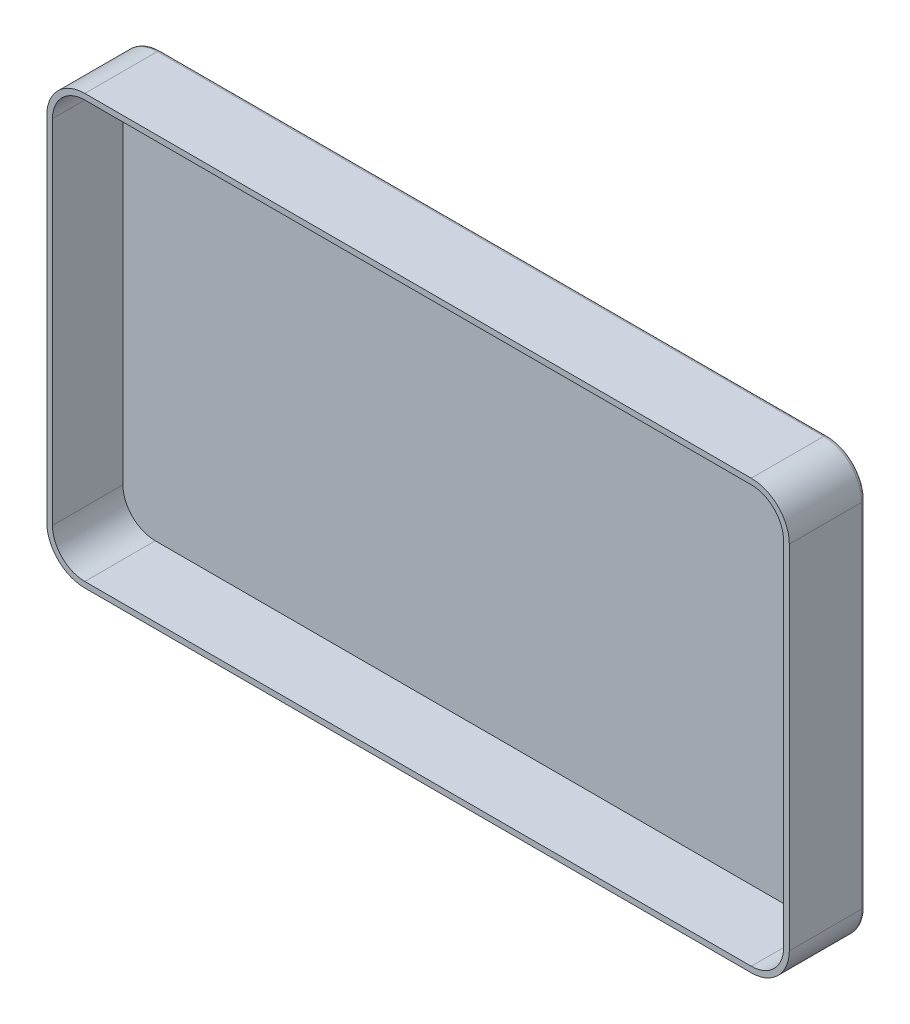
from build123d import *

# Parameters (mm, degrees)
SKETCH_1_W                     = 390
SKETCH_1_H                     = 225
EXTRUDE_1_DEPTH                = 40
FILLET_1_R                     = 20
SHELL_1_T                      = -3
FILLET_2_R                     = 2
SKETCH_2_R                     = 7.5
EXTRUDE_2_DEPTH                = 8
FILLET_3_R                     = 2
PATTERN_LINEAR_1_COUNT         = 2
PATTERN_LINEAR_1_PITCH         = 260
PATTERN_LINEAR_1_COUNT_DIR2    = 2
PATTERN_LINEAR_1_PITCH_DIR2    = 130
FILLET_3_OF_PATTERN_LINEAR_1_R = 2


with BuildPart() as part:
    # 草图1 → 凸台-拉伸1 (new body)
    with BuildSketch(Plane.XY):
        Rectangle(SKETCH_1_W, SKETCH_1_H)
    extrude(amount=EXTRUDE_1_DEPTH)

    # 圆角1
    fillet_1_edges = [part.edges().sort_by_distance(p)[0] for p in [
        (195, -112.5, 20),
        (-195, -112.5, 20),
        (-195, 112.5, 20),
        (195, 112.5, 20),
    ]]
    fillet(fillet_1_edges, radius=FILLET_1_R)

    # 抽壳1
    shell_1_openings = [part.faces().sort_by_distance(p)[0] for p in [
        (0, 0, 40),
    ]]
    offset(amount=SHELL_1_T, openings=shell_1_openings, kind=Kind.INTERSECTION)

    # 圆角2
    fillet_2_edges = [part.edges().sort_by_distance(p)[0] for p in [
        (195, 0, 0),
        (0, -112.5, 0),
        (-195, 0, 0),
        (0, 112.5, 0),
        (-189.142135624, -106.642135624, 0),
        (189.142135624, 106.642135624, 0),
        (-189.142135624, 106.642135624, 0),
        (189.142135624, -106.642135624, 0),
    ]]
    fillet(fillet_2_edges, radius=FILLET_2_R)

    # 草图2 → 凸台-拉伸2 (add)
    with BuildSketch(Plane(origin=(0, 0, 0), x_dir=(-1, 0, 0), z_dir=(0, 0, -1))):
        with Locations((-130, 65)):
            Circle(SKETCH_2_R)
    extrude_2 = extrude(amount=EXTRUDE_2_DEPTH)

    # 圆角3
    fillet_3_edges = [part.edges().sort_by_distance(p)[0] for p in [
        (137.5, 65, -8),
    ]]
    fillet(fillet_3_edges, radius=FILLET_3_R)

    # 阵列(线性)1: Extrude 2 2 × 2
    with Locations(*[(-i * PATTERN_LINEAR_1_PITCH, -j * PATTERN_LINEAR_1_PITCH_DIR2, 0) for i in range(PATTERN_LINEAR_1_COUNT) for j in range(PATTERN_LINEAR_1_COUNT_DIR2) if (i, j) != (0, 0)]):
        add(extrude_2)

    # 圆角3 of 阵列(线性)1
    fillet_3_of_pattern_linear_1_edges = [part.edges().sort_by_distance(p)[0] for p in [
        (137.5, -65, -8),
        (-122.5, 65, -8),
        (-122.5, -65, -8),
    ]]
    fillet(fillet_3_of_pattern_linear_1_edges, radius=FILLET_3_OF_PATTERN_LINEAR_1_R)


solid = part.part
